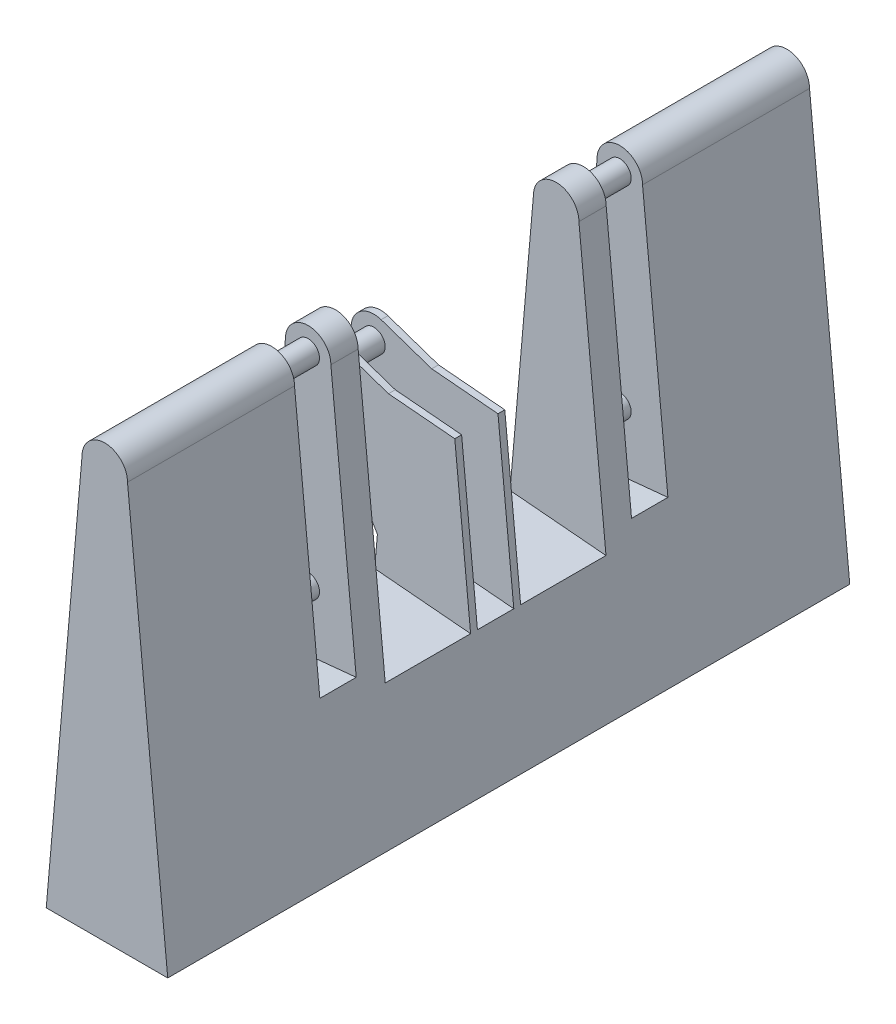
from build123d import *

# Parameters (mm, degrees)
SKETCH_1_5_R            = 100
SKETCH_1_5_R_2          = 50
BOSS_EXTRUDE1_DEPTH     = 3000
BOSS_EXTRUDE2_START     = -1390
SKETCH_1_4_R            = 100
SKETCH_1_4_R_2          = 50
BOSS_EXTRUDE2_DEPTH     = 30
SKETCH2_W               = 160
SKETCH2_H               = 1300
CUT_EXTRUDE1_DEPTH      = 3372.499629859
BOSS_EXTRUDE3_REACH     = 3411.07
SKETCH_1_5_2_R          = 50
SKETCH3_W               = 375.5
SKETCH3_H               = 1405.841341372
CUT_EXTRUDE2_DEPTH      = 3370.634545963
CUT_EXTRUDE3_DEPTH      = 3370.634545963
CUT_EXTRUDE4_DEPTH      = 3370.634545963
CUT_EXTRUDE4_DEPTH_BACK = 3370.634545963
SKETCH5_W               = 421.157999818
SKETCH5_H               = 173.673401987
SKETCH6_R               = 50
BOSS_EXTRUDE4_DEPTH     = 220
SKETCH7_R               = 50
BOSS_EXTRUDE5_DEPTH     = 1014.5


with BuildPart() as part:
    # Sketch 1_5 → Boss-Extrude1 (new body)
    # profile 1 of 3: a face of its own
    with BuildSketch(Plane.XY):
        with BuildLine():
            ThreePointArc((584.417791302, 1329.00950863), (484.417791302, 1229.00950863), (384.417791302, 1329.00950863))
            Line((384.417791302, 1329.00950863), (342.529038033, 850.218867874))
            Line((342.529038033, 850.218867874), (293.584845824, 290.784191003))
            Line((293.584845824, 290.784191003), (226.938196955, -470.99049137))
            Line((226.938196955, -470.99049137), (761.373330839, -470.99049137))
            Line((761.373330839, -470.99049137), (584.417791302, 1329.00950863))
        make_face()
    # profile 2 of 3: a face of its own
    with BuildSketch(Plane.XY):
        with Locations((484.417791302, 1329.00950863)):
            Circle(SKETCH_1_5_R)
        with Locations((484.417791302, 1329.00950863)):
            Circle(SKETCH_1_5_R_2, mode=Mode.SUBTRACT)
    # profile 3 of 3: a face of its own
    with BuildSketch(Plane.XY):
        with Locations((484.417791302, 1329.00950863)):
            Circle(SKETCH_1_5_R_2)
    extrude(amount=-BOSS_EXTRUDE1_DEPTH)

    # 草图1<4> → Boss-Extrude2 (add)
    # profile 1 of 2: a face of its own
    with BuildSketch(Plane.XY.offset(BOSS_EXTRUDE2_START)):
        with BuildLine():
            Line((293.584845824, 290.784191003), (342.529038033, 850.218867874))
            Line((342.529038033, 850.218867874), (120.005017386, 926.041198717))
            ThreePointArc((120.005017386, 926.041198717), (169.070315555, 889.586231815), (187.752156036, 831.385227248))
            ThreePointArc((187.752156036, 831.385227248), (114.3070167, 734.975479945), (1.855368534, 780.182279122))
            Line((1.855368534, 780.182279122), (293.584845824, 290.784191003))
        make_face()
    # profile 2 of 2: a face of its own
    with BuildSketch(Plane.XY.offset(BOSS_EXTRUDE2_START)):
        with Locations((87.752156036, 831.385227248)):
            Circle(SKETCH_1_4_R)
        with Locations((87.752156036, 831.385227248)):
            Circle(SKETCH_1_4_R_2, mode=Mode.SUBTRACT)
    boss_extrude2 = extrude(amount=-BOSS_EXTRUDE2_DEPTH)

    # Mirror1: Boss-Extrude2 across plane
    add(boss_extrude2.mirror(Plane.XY.offset(-1500)))

    # Sketch2 → Cut-Extrude1 (cut, symmetric)
    with BuildSketch(Plane(origin=(708.226185615, 69.624748217, 0), x_dir=(0, 0, -1), z_dir=(0.9952024531915172, 0.09783699280735358, 0))):
        with Locations((814.5, 775.344705163)):
            Rectangle(SKETCH2_W, SKETCH2_H)
    cut_extrude1 = extrude(amount=CUT_EXTRUDE1_DEPTH, both=True, mode=Mode.SUBTRACT)

    # Mirror2: Cut-Extrude1 across plane
    add(cut_extrude1.mirror(Plane.XY.offset(-1500)), mode=Mode.SUBTRACT)

    # Sketch 1_5 2 → Boss-Extrude3 (add, up to next)
    with BuildSketch(Plane.XY, mode=Mode.PRIVATE) as boss_extrude3_sk1:
        with Locations((484.417791302, 1329.00950863)):
            Circle(SKETCH_1_5_2_R)
    boss_extrude3_tool1 = extrude(boss_extrude3_sk1.sketch, amount=-BOSS_EXTRUDE3_REACH, mode=Mode.PRIVATE) - part.part
    add(boss_extrude3_tool1.solids().sort_by_distance((484.417791, 1329.009509, 0))[0])
    add(boss_extrude3_tool1.solids().sort_by_distance((484.417791, 1329.009509, 0))[1])

    # Sketch3 → Cut-Extrude2 (cut, symmetric)
    with BuildSketch(Plane(origin=(266.107666648, -23.281404109, 0), x_dir=(0, 0, 1), z_dir=(-0.9961946980917458, 0.0871557427476561, 0))):
        with Locations((-1202.25, 880.509090801)):
            Rectangle(SKETCH3_W, SKETCH3_H)
    cut_extrude2 = extrude(amount=CUT_EXTRUDE2_DEPTH, both=True, mode=Mode.SUBTRACT)

    # Mirror3: Cut-Extrude2 across plane
    add(cut_extrude2.mirror(Plane.XY.offset(-1500)), mode=Mode.SUBTRACT)

    # Sketch4 → Cut-Extrude3 (cut, through all)
    with BuildSketch(Plane(origin=(266.107666648, -23.281404109, 0), x_dir=(0, 0, 1), z_dir=(-0.9961946980917458, 0.0871557427476561, 0))):
        Polygon((-1672.587737226, 1602.596949433), (-1327.412262774, 1602.596949433), (-1327.412262774, 876.836901116), (-1420, 876.836901116), (-1420, 177.588420115), (-1580, 177.588420115), (-1580, 876.836901116), (-1672.587737226, 876.836901116), align=None)
    extrude(amount=-CUT_EXTRUDE3_DEPTH, mode=Mode.SUBTRACT)


with BuildPart() as cut_extrude3_piece_1:
    # of the separate pieces the step leaves, piece 1, a body of its own (cut_extrude3_pieces)
    add(part.part.solids().sort_by_distance((384.417791302, 1329.00950863, -3000))[0])

    # Sketch6 → Boss-Extrude4 (add)
    with BuildSketch(Plane.XY.offset(-1390)):
        with Locations((87.752156036, 831.385227248)):
            Circle(SKETCH6_R)
    extrude(amount=-BOSS_EXTRUDE4_DEPTH)

    # Sketch7 → Boss-Extrude5 (add)
    with BuildSketch(Plane.XY):
        with Locations((484.417791302, 439.00950863)):
            Circle(SKETCH7_R)
    boss_extrude5 = extrude(amount=-BOSS_EXTRUDE5_DEPTH)

    # Mirror4: Boss-Extrude5 across plane
    add(boss_extrude5.mirror(Plane.XY.offset(-1500)))


with BuildPart() as cut_extrude3_piece_2:
    # of the separate pieces the step leaves, piece 2, a body of its own (cut_extrude3_pieces)
    add(part.part.solids().sort_by_distance((385.937016001, 1346.374326397, -1390))[0])

    # Sketch5 → Cut-Extrude4 (cut, two sides: drawn at the far end of the back side and taken through both)
    with BuildSketch(Plane(origin=(266.107666648, -23.281404109, 0), x_dir=(0, 0, 1), z_dir=(-0.9961946980917458, 0.0871557427476561, 0)).offset(-CUT_EXTRUDE4_DEPTH_BACK)):
        with Locations((-1476.119907227, 1348.970668805)):
            Rectangle(SKETCH5_W, SKETCH5_H)
    extrude(amount=CUT_EXTRUDE4_DEPTH + CUT_EXTRUDE4_DEPTH_BACK, mode=Mode.SUBTRACT)


solid = cut_extrude3_piece_1.part
